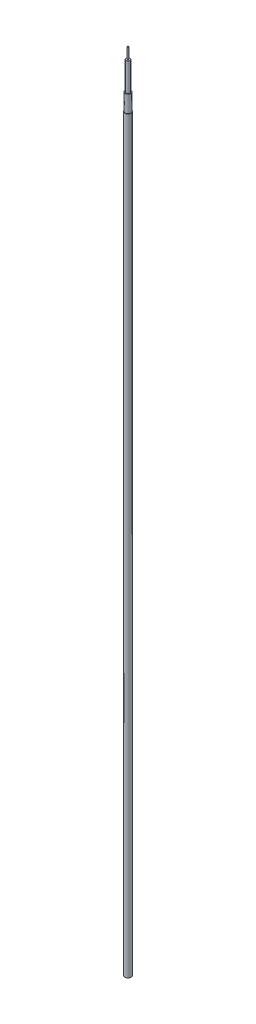
from build123d import *

# Parameters (mm, degrees)
SKETCH_1_R      = 0.565
EXTRUDE_1_DEPTH = 133
SKETCH_2_R      = 0.5
EXTRUDE_2_DEPTH = 3
SKETCH_3_R      = 0.35
EXTRUDE_3_DEPTH = 5
SKETCH_5_R      = 0.1
EXTRUDE_4_DEPTH = 2


with BuildPart() as part:
    # 草图1 → 凸台-拉伸1 (new body)
    with BuildSketch(Plane(origin=(0, 0, 0), x_dir=(1, 0, 0), z_dir=(0, 1, 0))):
        with Locations(Location((0, 0, 0), (0, 0, 270))):
            Circle(SKETCH_1_R)
    extrude(amount=EXTRUDE_1_DEPTH)

    # 草图2 → 凸台-拉伸2 (add)
    with BuildSketch(Plane(origin=(0, 133, 0), x_dir=(1, 0, 0), z_dir=(0, 1, 0))):
        with Locations(Location((0, 0, 0), (0, 0, 270))):
            Circle(SKETCH_2_R)
    extrude(amount=EXTRUDE_2_DEPTH)

    # 草图3 → 凸台-拉伸3 (add)
    with BuildSketch(Plane(origin=(0, 136, 0), x_dir=(1, 0, 0), z_dir=(0, 1, 0))):
        with Locations(Location((0, 0, 0), (0, 0, 270))):
            Circle(SKETCH_3_R)
    extrude(amount=EXTRUDE_3_DEPTH)

    # 草图5 → 凸台-拉伸4 (add)
    with BuildSketch(Plane(origin=(0, 141, 0), x_dir=(1, 0, 0), z_dir=(0, 1, 0))):
        with Locations(Location((0, 0, 0), (0, 0, 270))):
            Circle(SKETCH_5_R)
    extrude(amount=EXTRUDE_4_DEPTH)


solid = part.part
